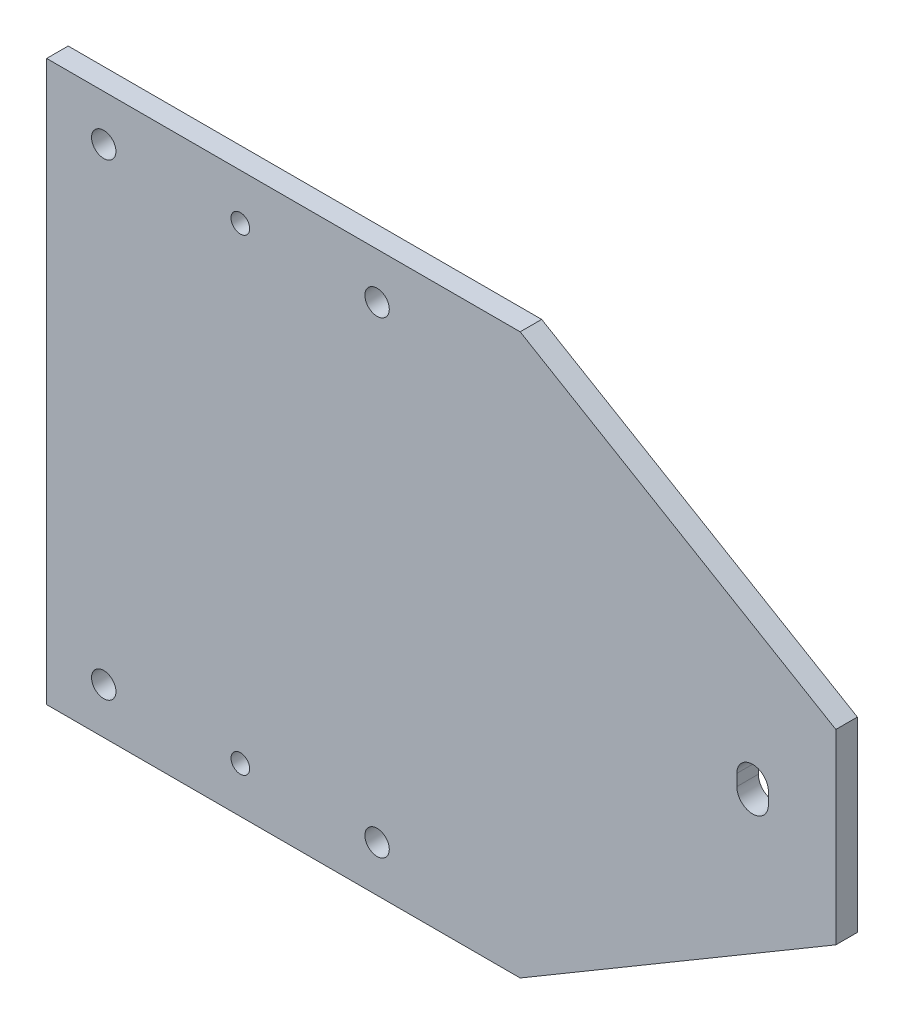
from build123d import *

# Parameters (mm, degrees)
SKETCH_1_W          = 550
SKETCH_1_H          = 390
EXTRUDE_1_DEPTH     = 15
SKETCH_2_R          = 8.5
SKETCH_2_R_2        = 6.5
CUT_EXTRUDE_1_DEPTH = 15


with BuildPart() as part:
    # 草图1 → 凸台-拉伸1 (new body)
    with BuildSketch(Plane.XY):
        Rectangle(SKETCH_1_W, SKETCH_1_H)
    extrude(amount=EXTRUDE_1_DEPTH)

    # 草图2 → 切除-拉伸1 (cut)
    with BuildSketch(Plane.XY.offset(15)):
        with Locations((-235.2, 163)):
            Circle(SKETCH_2_R)
        with Locations((-235.2, -163)):
            Circle(SKETCH_2_R)
        with Locations((-140, -163)):
            Circle(SKETCH_2_R_2)
        with Locations((-44.7, -163)):
            Circle(SKETCH_2_R)
        with Locations((-140, 163)):
            Circle(SKETCH_2_R_2)
        with Locations((-44.7, 163)):
            Circle(SKETCH_2_R)
        Polygon((55, 195), (275, 65), (275, 195), align=None)
        Polygon((55, -195), (275, -65), (275, -195), align=None)
        with BuildLine():
            Line((228, 4), (228, -4))
            ThreePointArc((228, -4), (217, -15), (206, -4))
            Line((206, -4), (206, 4))
            ThreePointArc((206, 4), (217, 15), (228, 4))
        make_face()
    extrude(amount=-CUT_EXTRUDE_1_DEPTH, mode=Mode.SUBTRACT)


solid = part.part
